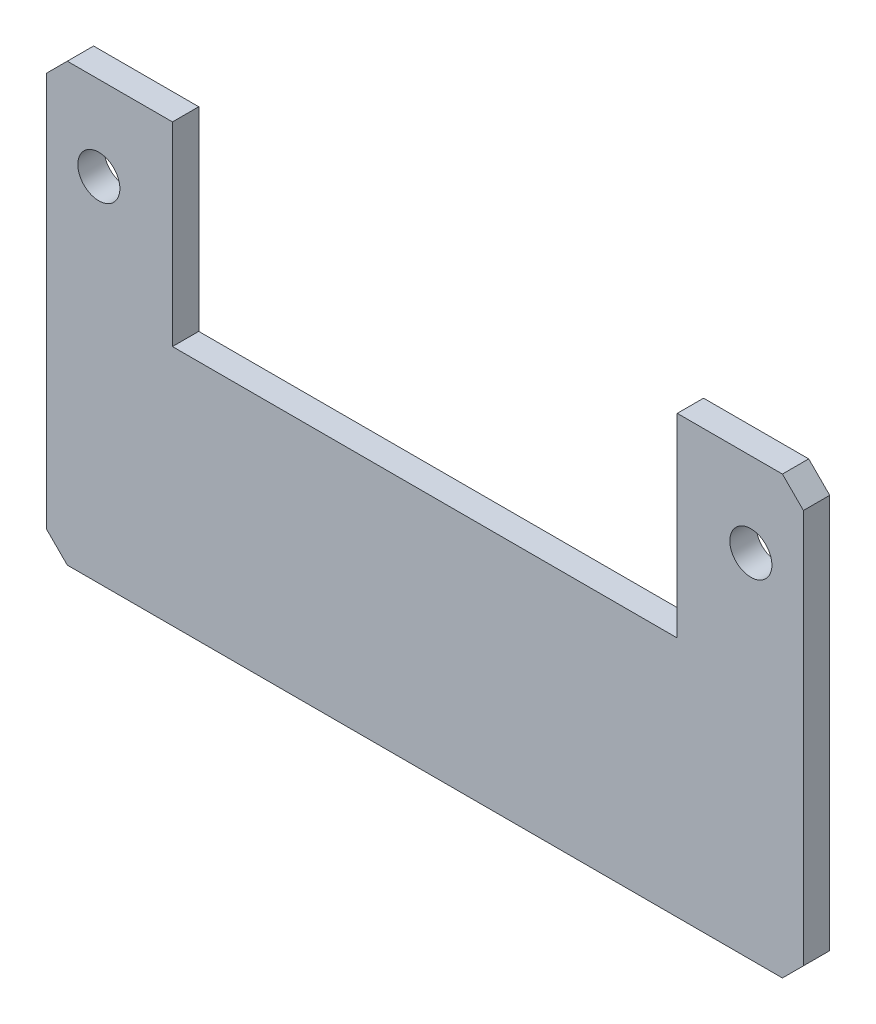
SolidWorks part; units mm, degrees
ref_plane "Front Plane" through (0, 0, 0) normal (0, 0, 1) x (1, 0, 0)
ref_plane "Top Plane" through (0, 0, 0) normal (0, 1, 0) x (1, 0, 0)
ref_plane "Right Plane" through (0, 0, 0) normal (1, 0, 0) x (0, 0, -1)
sketch "Sketch1" plane through (0, 0, 0) normal (0, 0, 1) x (1, 0, 0)
  line L0 (360, -415) -> (360, 0) construction
  line L1 (0, 0) -> (720, 0)
  line L2 (0, 0) -> (0, -415)
  line L3 (0, -415) -> (720, -415)
  line L4 (720, 0) -> (720, -415)
  line L5 (600, -185) -> (120, -185)
  line L6 (600, -185) -> (600, 0)
  line L7 (600, 0) -> (120, 0)
  line L8 (120, -185) -> (120, 0)
  line L9 (600, -185) -> (120, 0) construction
  line L10 (600, 0) -> (120, -185) construction
  circle A0 centre (50, -80) radius 20
  circle A1 centre (670, -80) radius 20
  point P5 (360, -92.5)
  dimension "D7" = 40
  dimension "D8" = 80
  dimension "D10" = 40
  dimension "D1" = 720
  dimension "D2" = 415
  dimension "D3" = 480
  dimension "D4" = 185
  dimension "D5" = 50
  dimension "D6" = 80
  dimension "D9" = 50
extrude "Boss-Extrude1" add sketch "Sketch1" along normal blind 25 contours L5 L8 L1 L2 L3 L4 L6
chamfer "Chamfer1" distance 20 angle 45 4 edges at (0, 0, 12.5) (0, -415, 12.5) (720, -415, 12.5) (720, 0, 12.5)
